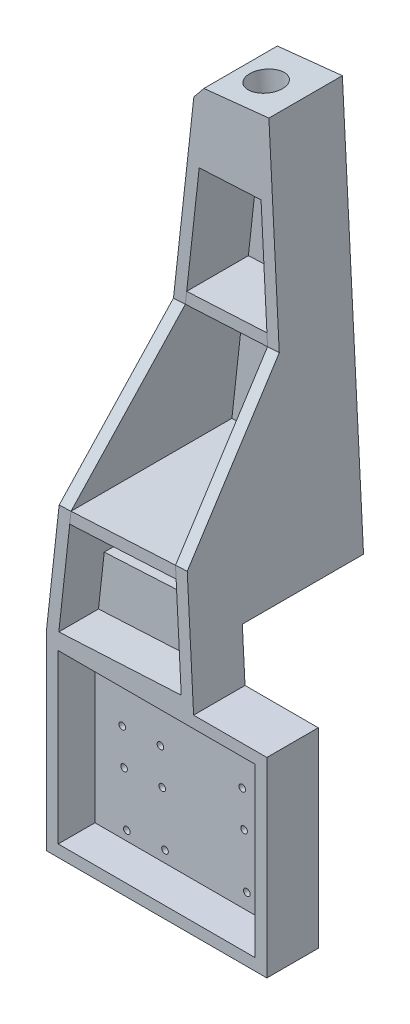
from build123d import *

# Parameters (mm, degrees)
SKETCH_1_W           = 300
SKETCH_1_H           = 260
EXTRUDE_1_DEPTH      = 70
SHELL_1_T            = -16
EXTRUDE_2_DEPTH      = 200
EXTRUDE_8_REACH      = 660.101
SKETCH_19_W          = 200
SKETCH_19_H          = 70
CUT_EXTRUDE_1_DEPTH  = 807.862444051
CUT_EXTRUDE_4_REACH  = 791.41
CUT_EXTRUDE_8_DEPTH  = 100
EXTRUDE_3_DEPTH      = 84
EXTRUDE_4_DEPTH      = 219
EXTRUDE_5_DEPTH      = 4
CUT_EXTRUDE_10_REACH = 917.388
SKETCH_16_R          = 22.5
CHAMFER_1_SIZE       = 12
CHAMFER_1_SIZE2      = 15.70753971
SKETCH_21_R          = 4.5
CUT_EXTRUDE_12_DEPTH = 20


with BuildPart() as part:
    # 草图1 → 凸台-拉伸1 (new body)
    with BuildSketch(Plane.XY):
        Rectangle(SKETCH_1_W, SKETCH_1_H)
    extrude(amount=EXTRUDE_1_DEPTH)

    # 抽壳1
    shell_1_openings = [part.faces().sort_by_distance(p)[0] for p in [
        (0, 0, 70),
    ]]
    offset(amount=SHELL_1_T, openings=shell_1_openings, kind=Kind.INTERSECTION)

    # 凸台-拉伸8: up to this face of the body (flat: up to its plane)
    extrude_8_end = Plane(part.part.faces().sort_by_distance((0, 130, 35))[0])
    # 草图19 → 凸台-拉伸8 (add, up to the picked face)
    with BuildSketch(Plane(origin=(-7.20520796, 137.483557944, 0), x_dir=(0.998629534754574, 0.052335956242943966, 0), z_dir=(0.052335956242943966, -0.998629534754574, 0)), mode=Mode.PRIVATE) as extrude_8_sk1:
        with Locations((-42.990755902, 35)):
            Rectangle(SKETCH_19_W, SKETCH_19_H)
    extrude_8_tool1 = split(extrude(extrude_8_sk1.sketch, amount=EXTRUDE_8_REACH, mode=Mode.PRIVATE), bisect_by=extrude_8_end, keep=Keep.BOTH, mode=Mode.PRIVATE)


with BuildPart() as body_2:
    # 草图2 → 凸台-拉伸2 (new body)
    with BuildSketch(Plane(origin=(-141.972841921, -23.167300518, 0), x_dir=(0, 0, 1), z_dir=(0.998629534754574, 0.05233595624294396, 0))):
        Polygon((-165, -213.37749905), (0, -213.37749905), (0, -153.37749905), (70, -153.37749905), (70, -308.37749905), (-65, -493.87749905), (-65, -763.87749905), (-165, -763.87749905), align=None)
    extrude(amount=EXTRUDE_2_DEPTH)


with BuildPart() as part_1:
    add(part.part)

    add(body_2.part)  # 凸台-拉伸8 merges body 2
    add(extrude_8_tool1.solids().sort_by(Axis((-50.137047, 135.233596, 35), (0.052335956242943966, -0.998629534754574, 0)))[0])

    # 草图3 → 切除-拉伸1 (cut, through all)
    with BuildSketch(Plane(origin=(0, 0, -165), x_dir=(-1, 0, 0), z_dir=(0, 0, -1))):
        Polygon((150, 130), (82.088147811, 744.896926592), (181.951101286, 739.663330968), align=None)
    extrude(amount=-CUT_EXTRUDE_1_DEPTH, mode=Mode.SUBTRACT)

    # 切除-拉伸4: up to this plane
    cut_extrude_4_end = Plane(origin=(-134.096699763, 128.243571356, 70), z_dir=(0.993956264793354, -0.10977679025205724, 0))
    # 草图6 → 切除-拉伸4 (cut, up to the surface)
    with BuildSketch(Plane(origin=(40.953042355, 2.146258005, 0), x_dir=(0, 0, -1), z_dir=(0.998629534754574, 0.052335956242943994, 0)), mode=Mode.PRIVATE) as cut_extrude_4_sk1:
        Polygon((55, 647.190677098), (149, 647.190677098), (149, 213.672232955), (-16, 213.672232955), (-16, 143.190677098), (-80, 143.190677098), (-80, 308.190677098), (55, 513.190677098), align=None)
    cut_extrude_4_tool1 = split(extrude(cut_extrude_4_sk1.sketch, amount=-CUT_EXTRUDE_4_REACH, mode=Mode.PRIVATE), bisect_by=cut_extrude_4_end, keep=Keep.BOTH, mode=Mode.PRIVATE)
    add(cut_extrude_4_tool1.solids().sort_by_distance((21.372387, 375.767411, -54.53636))[0], mode=Mode.SUBTRACT)

    # 草图7 → 切除-拉伸8 (cut)
    with BuildSketch(Plane(origin=(159.725965218, 1446.779693797, -165), x_dir=(-0.9759167619387475, 0.2181432413965424, 0), z_dir=(0, 0, 1))):
        Polygon((82.87946426, 737.729271863), (82.291888761, 743.053550343), (-13.43679242, 710.837289802), align=None)
    extrude(amount=CUT_EXTRUDE_8_DEPTH, mode=Mode.SUBTRACT)

    # 草图11 → 凸台-拉伸5 (add)
    with BuildSketch(Plane.XY.offset(16)):
        Polygon((134, 114), (134, -114), (-134, -114), (-134, 114), (-5.07381302, 114), align=None)
    extrude(amount=EXTRUDE_5_DEPTH)

    # 切除-拉伸10: up to this plane
    cut_extrude_10_end = Plane(origin=(-690.839974359, 611.873457737, -55), z_dir=(-0.05233595624294398, 0.9986295347545739, 0))
    # 草图16 → 切除-拉伸10 (cut, up to the surface)
    with BuildSketch(Plane(origin=(-84.138527977, 739.41899922, 0), x_dir=(-0.9945218953682742, -0.10452846326764542, 0), z_dir=(0.10452846326764542, -0.9945218953682742, 0)), mode=Mode.PRIVATE) as cut_extrude_10_sk1:
        with Locations((-51.470404609, 112)):
            Circle(SKETCH_16_R)
    cut_extrude_10_tool1 = split(extrude(cut_extrude_10_sk1.sketch, amount=CUT_EXTRUDE_10_REACH, mode=Mode.PRIVATE), bisect_by=cut_extrude_10_end, keep=Keep.BOTH, mode=Mode.PRIVATE)
    add(cut_extrude_10_tool1.solids().sort_by_distance((-32.950084, 744.799122, -112))[0], mode=Mode.SUBTRACT)

    # 倒角1
    chamfer_1_edges = [part_1.edges().sort_by_distance(p)[0] for p in [
        (-82.676178398, 739.572698355, -115),
    ]]
    chamfer_1_side = [part_1.faces().sort_by_distance(p)[0] for p in [
        (-81.262631859, 739.721268083, -115),
    ]]
    chamfer(chamfer_1_edges, length=CHAMFER_1_SIZE, length2=CHAMFER_1_SIZE2, reference=chamfer_1_side[0])

    # 草图21 → 切除-拉伸12 (cut)
    with BuildSketch(Plane(origin=(0, 0, 0), x_dir=(-1, 0, 0), z_dir=(0, 0, -1))):
        with Locations((90.556644666, -101.205834721)):
            Circle(SKETCH_21_R)
        with Locations((38.627908859, -98.484364996)):
            Circle(SKETCH_21_R)
        with Locations((94.324833516, -29.304508218)):
            Circle(SKETCH_21_R)
        with Locations((42.396097708, -26.583038494)):
            Circle(SKETCH_21_R)
        with Locations((96.836959422, 18.629709456)):
            Circle(SKETCH_21_R)
        with Locations((44.908223614, 21.351179181)):
            Circle(SKETCH_21_R)
        with Locations((48.676412464, 93.252505683)):
            Circle(SKETCH_21_R)
        with Locations((100.605148271, 90.531035958)):
            Circle(SKETCH_21_R)
        with Locations((-114.619489059, 101.810481248)):
            Circle(SKETCH_21_R)
        with Locations((-62.690753252, 99.089011523)):
            Circle(SKETCH_21_R)
        with Locations((-118.387677909, 29.909154746)):
            Circle(SKETCH_21_R)
        with Locations((-66.458942101, 27.187685021)):
            Circle(SKETCH_21_R)
        with Locations((-120.899803815, -18.025062929)):
            Circle(SKETCH_21_R)
        with Locations((-68.971068007, -20.746532653)):
            Circle(SKETCH_21_R)
        with Locations((-124.667992664, -89.926389431)):
            Circle(SKETCH_21_R)
        with Locations((-72.739256857, -92.647859156)):
            Circle(SKETCH_21_R)
    extrude(amount=-CUT_EXTRUDE_12_DEPTH, mode=Mode.SUBTRACT)


with BuildPart() as body_2_2:
    # 草图9 → 凸台-拉伸3 (new body)
    with BuildSketch(Plane.XY.offset(-65)):
        Polygon((-95.931870058, 473.800874433), (-94.152034456, 489.9161092), (15.090065994, 495.641245089), (15.927441294, 479.663172533), align=None)
    extrude(amount=-EXTRUDE_3_DEPTH)


with BuildPart() as body_3:
    # 草图10 → 凸台-拉伸4 (new body)
    with BuildSketch(Plane.XY.offset(70)):
        Polygon((25.635761177, 294.417393836), (-116.566839069, 286.964871348), (-118.346674671, 270.849636581), (26.473136477, 278.43932128), align=None)
    extrude(amount=-EXTRUDE_4_DEPTH)


solid = Compound([part_1.part, body_2_2.part, body_3.part])
